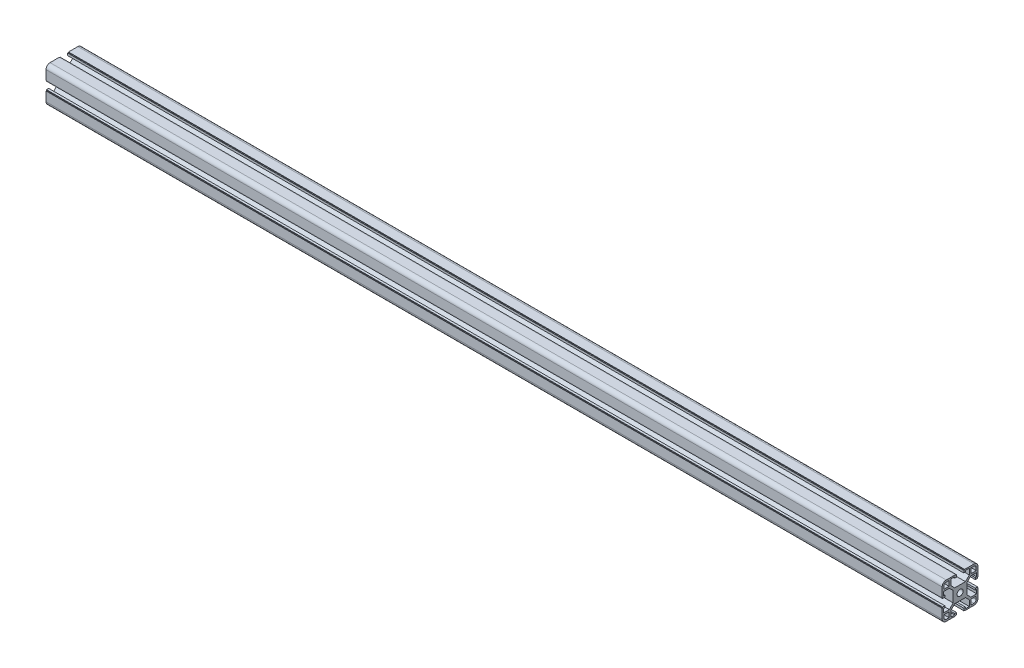
from build123d import *

# Parameters (mm, degrees)
SKETCH1_R                                 = 3.4
ALUMINIUM_PROFILE_40_X_40B_X_R4_5_1_DEPTH = 1000


with BuildPart() as part:
    # Sketch1 → Aluminium profile 40 X 40B X R4.5(1) (new body)
    with BuildSketch(Plane.YZ.offset(-484.974958264)):
        with BuildLine():
            Line((-5.1, 20), (-5.1, 19.5))
            Line((-5.1, 19.5), (-4.1, 19.5))
            Line((-4.1, 19.5), (-4.1, 17))
            Line((-4.1, 17), (-6.1, 17))
            Line((-6.1, 17), (-6.1, 18.5))
            Line((-6.1, 18.5), (-10.3, 18.5))
            Line((-10.3, 18.5), (-10.3, 12))
            Line((-10.3, 12), (-6, 7.7))
            Line((-6, 7.7), (6, 7.7))
            Line((6, 7.7), (10.3, 12))
            Line((10.3, 12), (10.3, 18.5))
            Line((10.3, 18.5), (6.1, 18.5))
            Line((6.1, 18.5), (6.1, 17))
            Line((6.1, 17), (4.1, 17))
            Line((4.1, 17), (4.1, 19.5))
            Line((4.1, 19.5), (5.1, 19.5))
            Line((5.1, 19.5), (5.1, 20))
            Line((5.1, 20), (15.5, 20))
            ThreePointArc((15.5, 20), (18.681980515, 18.681980515), (20, 15.5))
            Line((20, 15.5), (20, 5.1))
            Line((20, 5.1), (19.5, 5.1))
            Line((19.5, 5.1), (19.5, 4.1))
            Line((19.5, 4.1), (17, 4.1))
            Line((17, 4.1), (17, 6.1))
            Line((17, 6.1), (18.5, 6.1))
            Line((18.5, 6.1), (18.5, 10.3))
            Line((18.5, 10.3), (12, 10.3))
            Line((12, 10.3), (7.7, 6))
            Line((7.7, 6), (7.7, -6))
            Line((7.7, -6), (12, -10.3))
            Line((12, -10.3), (18.5, -10.3))
            Line((18.5, -10.3), (18.5, -6.1))
            Line((18.5, -6.1), (17, -6.1))
            Line((17, -6.1), (17, -4.1))
            Line((17, -4.1), (19.5, -4.1))
            Line((19.5, -4.1), (19.5, -5.1))
            Line((19.5, -5.1), (20, -5.1))
            Line((20, -5.1), (20, -15.5))
            ThreePointArc((20, -15.5), (18.681980515, -18.681980515), (15.5, -20))
            Line((15.5, -20), (5.1, -20))
            Line((5.1, -20), (5.1, -19.5))
            Line((5.1, -19.5), (4.1, -19.5))
            Line((4.1, -19.5), (4.1, -17))
            Line((4.1, -17), (6.1, -17))
            Line((6.1, -17), (6.1, -18.5))
            Line((6.1, -18.5), (10.3, -18.5))
            Line((10.3, -18.5), (10.3, -12))
            Line((10.3, -12), (6, -7.7))
            Line((6, -7.7), (-6, -7.7))
            Line((-6, -7.7), (-10.3, -12))
            Line((-10.3, -12), (-10.3, -18.5))
            Line((-10.3, -18.5), (-6.1, -18.5))
            Line((-6.1, -18.5), (-6.1, -17))
            Line((-6.1, -17), (-4.1, -17))
            Line((-4.1, -17), (-4.1, -19.5))
            Line((-4.1, -19.5), (-5.1, -19.5))
            Line((-5.1, -19.5), (-5.1, -20))
            Line((-5.1, -20), (-15.5, -20))
            ThreePointArc((-15.5, -20), (-18.681980515, -18.681980515), (-20, -15.5))
            Line((-20, -15.5), (-20, -5.1))
            Line((-20, -5.1), (-19.5, -5.1))
            Line((-19.5, -5.1), (-19.5, -4.1))
            Line((-19.5, -4.1), (-17, -4.1))
            Line((-17, -4.1), (-17, -6.1))
            Line((-17, -6.1), (-18.5, -6.1))
            Line((-18.5, -6.1), (-18.5, -10.3))
            Line((-18.5, -10.3), (-12, -10.3))
            Line((-12, -10.3), (-7.7, -6))
            Line((-7.7, -6), (-7.7, 6))
            Line((-7.7, 6), (-12, 10.3))
            Line((-12, 10.3), (-18.5, 10.3))
            Line((-18.5, 10.3), (-18.5, 6.1))
            Line((-18.5, 6.1), (-17, 6.1))
            Line((-17, 6.1), (-17, 4.1))
            Line((-17, 4.1), (-19.5, 4.1))
            Line((-19.5, 4.1), (-19.5, 5.1))
            Line((-19.5, 5.1), (-20, 5.1))
            Line((-20, 5.1), (-20, 15.5))
            ThreePointArc((-20, 15.5), (-18.681980515, 18.681980515), (-15.5, 20))
            Line((-15.5, 20), (-5.1, 20))
        make_face()
        Circle(SKETCH1_R, mode=Mode.SUBTRACT)
        with BuildLine():
            Line((12.3, 18), (15.5, 18))
            ThreePointArc((15.5, 18), (17.267766953, 17.267766953), (18, 15.5))
            Line((18, 15.5), (18, 12.3))
            Line((18, 12.3), (12.3, 12.3))
            Line((12.3, 12.3), (12.3, 18))
        make_face(mode=Mode.SUBTRACT)
        with BuildLine():
            Line((-15.5, 18), (-12.3, 18))
            Line((-12.3, 18), (-12.3, 12.3))
            Line((-12.3, 12.3), (-18, 12.3))
            Line((-18, 12.3), (-18, 15.5))
            ThreePointArc((-18, 15.5), (-17.267766953, 17.267766953), (-15.5, 18))
        make_face(mode=Mode.SUBTRACT)
        with BuildLine():
            Line((-18, -12.3), (-12.3, -12.3))
            Line((-12.3, -12.3), (-12.3, -18))
            Line((-12.3, -18), (-15.5, -18))
            ThreePointArc((-15.5, -18), (-17.267766953, -17.267766953), (-18, -15.5))
            Line((-18, -15.5), (-18, -12.3))
        make_face(mode=Mode.SUBTRACT)
        with BuildLine():
            Line((12.3, -12.3), (18, -12.3))
            Line((18, -12.3), (18, -15.5))
            ThreePointArc((18, -15.5), (17.267766953, -17.267766953), (15.5, -18))
            Line((15.5, -18), (12.3, -18))
            Line((12.3, -18), (12.3, -12.3))
        make_face(mode=Mode.SUBTRACT)
    extrude(amount=ALUMINIUM_PROFILE_40_X_40B_X_R4_5_1_DEPTH)


solid = part.part
